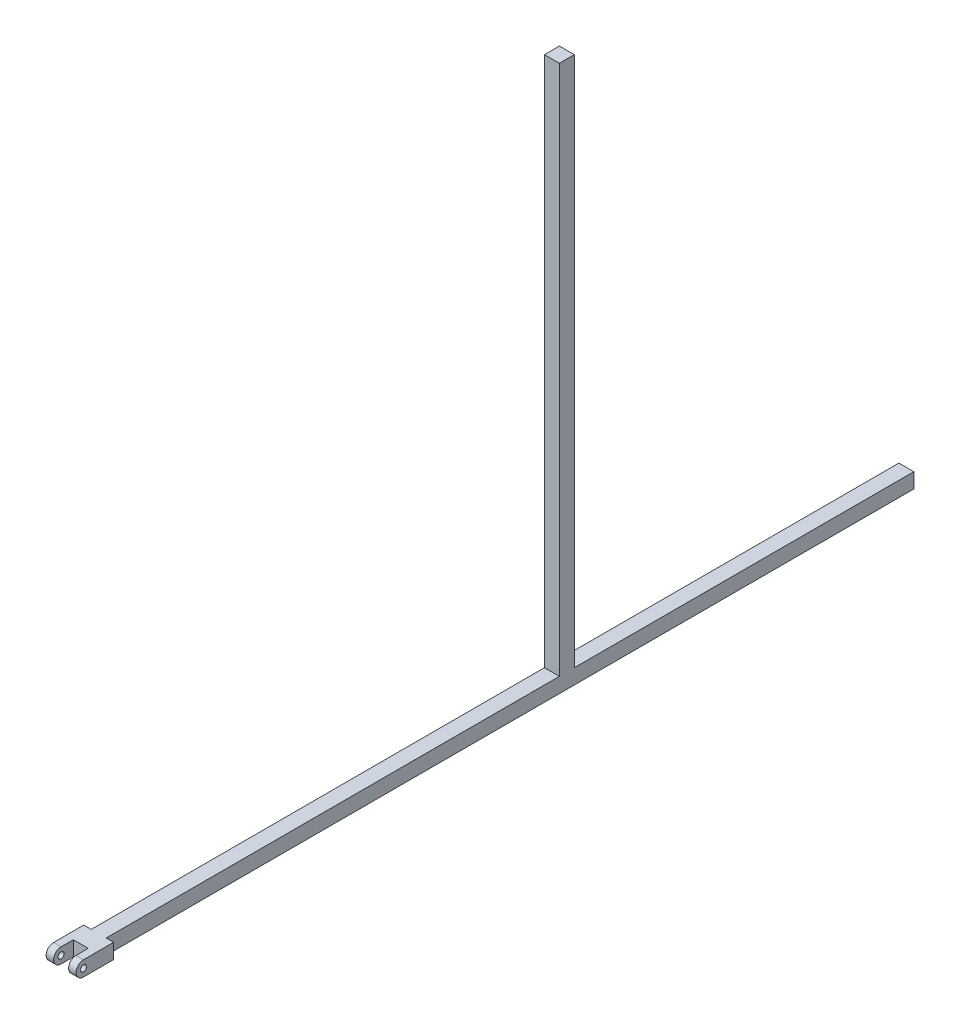
from build123d import *

# Parameters (mm, degrees)
SKETCH1_W               = 5
SKETCH1_H               = 5
BOSS_EXTRUDE1_DEPTH     = 270
SKETCH2_W               = 10
SKETCH2_H               = 5
BOSS_EXTRUDE2_DEPTH     = 18
SKETCH3_W               = 5
SKETCH3_H               = 19.358131828
CUT_EXTRUDE1_DEPTH      = 12
CUT_EXTRUDE2_DEPTH      = 289.18440277
CUT_EXTRUDE2_DEPTH_BACK = 289.18440277
SKETCH4_R               = 1
SKETCH5_W               = 5
SKETCH5_H               = 5
BOSS_EXTRUDE3_DEPTH     = 180


with BuildPart() as part:
    # Sketch1 → Boss-Extrude1 (new body)
    with BuildSketch(Plane.XY):
        Rectangle(SKETCH1_W, SKETCH1_H)
    extrude(amount=BOSS_EXTRUDE1_DEPTH)

    # Sketch2 → Boss-Extrude2 (add)
    with BuildSketch(Plane.XY.offset(270)):
        Rectangle(SKETCH2_W, SKETCH2_H)
    extrude(amount=BOSS_EXTRUDE2_DEPTH)

    # Sketch3 → Cut-Extrude1 (cut)
    with BuildSketch(Plane.XY.offset(288)):
        Rectangle(SKETCH3_W, SKETCH3_H)
    extrude(amount=-CUT_EXTRUDE1_DEPTH, mode=Mode.SUBTRACT)

    # Sketch4 → Cut-Extrude2 (cut, two sides: drawn at the far end of the back side and taken through both)
    with BuildSketch(Plane(origin=(5, 0, 0), x_dir=(0, 0, -1), z_dir=(1, 0, 0)).offset(-CUT_EXTRUDE2_DEPTH_BACK)):
        with Locations(Location((-280.07674021, 0, 0), (0, 0, 90))):
            Circle(SKETCH4_R)
        with BuildLine():
            Line((-280.07674021, 2.5), (-280.07674021, 12.098504892))
            Line((-280.07674021, 12.098504892), (-285.8811548, 12.098504892))
            Line((-285.8811548, 12.098504892), (-318.827178265, -19.142217328))
            Line((-318.827178265, -19.142217328), (-280.07674021, -2.5))
            ThreePointArc((-280.07674021, -2.5), (-282.57674021, 0), (-280.07674021, 2.5))
        make_face()
    extrude(amount=CUT_EXTRUDE2_DEPTH + CUT_EXTRUDE2_DEPTH_BACK, mode=Mode.SUBTRACT)

    # Sketch5 → Boss-Extrude3 (add)
    with BuildSketch(Plane(origin=(0, 0, 0), x_dir=(1, 0, 0), z_dir=(0, 1, 0))):
        with Locations((0, -116)):
            Rectangle(SKETCH5_W, SKETCH5_H)
    extrude(amount=BOSS_EXTRUDE3_DEPTH)


solid = part.part
